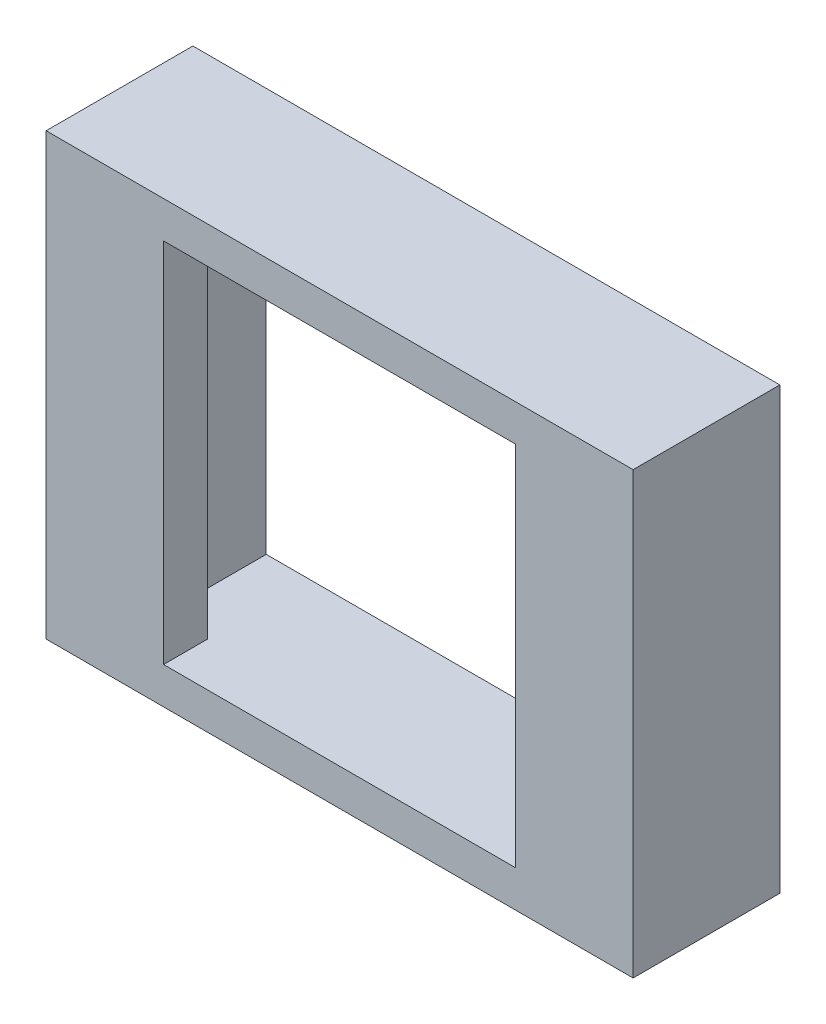
from build123d import *

# Parameters (mm, degrees)
SKETCH_1_W          = 80
SKETCH_1_H          = 60
EXTRUDE_1_DEPTH     = 20
CUT_EXTRUDE_1_REACH = 55.852
SKETCH_2_W          = 48
SKETCH_2_H          = 50
SKETCH_3_W          = 60
SKETCH_3_H          = 50
CUT_EXTRUDE_2_DEPTH = 14


with BuildPart() as part:
    # 草图1 → 凸台-拉伸1 (new body)
    with BuildSketch(Plane.XY):
        Rectangle(SKETCH_1_W, SKETCH_1_H)
    extrude(amount=EXTRUDE_1_DEPTH)

    # 草图2 → 切除-拉伸1 (cut, up to next)
    with BuildSketch(Plane.XY.offset(20), mode=Mode.PRIVATE) as cut_extrude_1_sk1:
        Rectangle(SKETCH_2_W, SKETCH_2_H)
    cut_extrude_1_tool1 = extrude(cut_extrude_1_sk1.sketch, amount=-CUT_EXTRUDE_1_REACH, mode=Mode.PRIVATE) & part.part
    add(cut_extrude_1_tool1.solids().sort_by_distance((0, 0, 20))[0], mode=Mode.SUBTRACT)

    # 草图3 → 切除-拉伸2 (cut)
    with BuildSketch(Plane(origin=(0, 0, 0), x_dir=(-1, 0, 0), z_dir=(0, 0, -1))):
        Rectangle(SKETCH_3_W, SKETCH_3_H)
    extrude(amount=-CUT_EXTRUDE_2_DEPTH, mode=Mode.SUBTRACT)


solid = part.part
